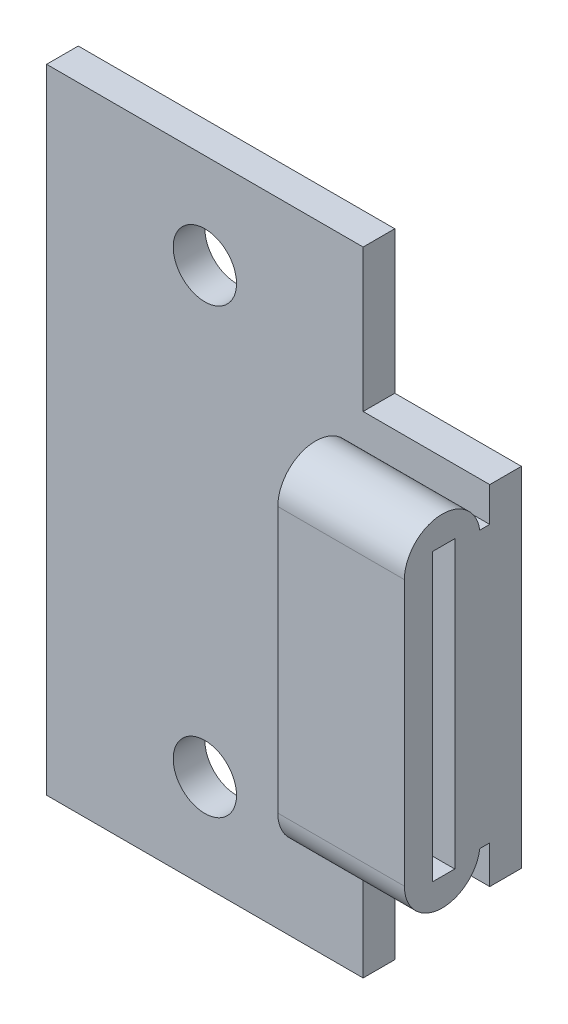
SolidWorks part; units mm, degrees
ref_plane "Front Plane" through (0, 0, 0) normal (0, 0, 1) x (1, 0, 0)
ref_plane "Top Plane" through (0, 0, 0) normal (0, 1, 0) x (1, 0, 0)
ref_plane "Right Plane" through (0, 0, 0) normal (1, 0, 0) x (0, 0, -1)
other "Configuration Table"
sketch "Sketch1" plane through (0, 0, 0) normal (0, 0, 1) x (1, 0, 0)
  line L0 (0, 7) -> (0, -7) construction
  line L1 (-5, 10) -> (5, 10)
  line L2 (-5, 10) -> (-5, -10)
  line L3 (-5, -10) -> (5, -10)
  line L4 (5, 10) -> (5, 5.5)
  line L5 (-5, 10) -> (5, -10) construction
  line L6 (-5, -10) -> (5, 10) construction
  line L11 (9, 5.5) -> (9, -5.5)
  line L12 (1, 5.5) -> (9, -5.5) construction
  line L13 (1, -5.5) -> (9, 5.5) construction
  line L14 (5, 5.5) -> (9, 5.5)
  line L15 (5, -5.5) -> (5, -10)
  line L16 (5, -5.5) -> (9, -5.5)
  circle A4 centre (0, 7) radius 1
  circle A5 centre (0, -7) radius 1
  point P0 (0, 0)
  point P6 (0, 0)
  point P11 (5, 0)
  dimension "D5" = 7
  dimension "D6" = 2
  dimension "D7" = 2
  dimension "D1" = 10
  dimension "D2" = 20
  dimension "D3" = 14
  dimension "D4" = 5
  dimension "D8" = 11
  dimension "D9" = 4
extrude "Boss-Extrude1" add sketch "Sketch1" along normal blind 1
sketch "Sketch2" plane through (0, 0, 1) normal (0, 0, 1) x (1, 0, 0)
  line L0 (5, 5.5) -> (5, 10) construction
  line L1 (9, 5.5) -> (5, 5.5)
  line L2 (9, 5.5) -> (9, -5.5)
  line L3 (9, -5.5) -> (5, -5.5)
  line L4 (5, 5.5) -> (5, -5.5)
  line L5 (9, 5.5) -> (5, -5.5) construction
  line L6 (9, -5.5) -> (5, 5.5) construction
  line L7 (9, -5.5) -> (9, 5.5) construction
  line L8 (9, 5.5) -> (5, 5.5) construction
  point P0 (7, 0)
extrude "Boss-Extrude2" add sketch "Sketch2" along normal blind 3
sketch "Sketch3" plane through (9, 0, 0) normal (1, 0, 0) x (0, 0, -1)
  line L0 (-2.5, 5.5) -> (-2.5, -5.5) construction
  line L1 (-4, 5.5) -> (0, 5.5) construction
  line L2 (-4, -5.5) -> (0, -5.5) construction
  line L3 (-4, -5.5) -> (-4, 5.5) construction
  line L4 (-2.5, 4.2479) -> (-2.5, -4.1397) construction
  line L5 (-1.3037, 4.2479) -> (-1.3037, -4.1397)
  line L6 (-3.6963, 4.2479) -> (-3.6963, -4.1397)
  line L8 (-1, -5.5) -> (-4, -5.5)
  line L9 (-1, -5.5) -> (-1, 5.5)
  line L10 (-1, 5.5) -> (-4, 5.5)
  line L11 (-4, -5.5) -> (-4, 5.5)
  line L12 (-1, -5.5) -> (-4, 5.5) construction
  line L13 (-1, 5.5) -> (-4, -5.5) construction
  arc A0 (-1.3037, 4.2479) -> (-3.6963, 4.2479) centre (-2.5, 4.2479) ccw
  arc A1 (-3.6963, -4.1397) -> (-1.3037, -4.1397) centre (-2.5, -4.1397) ccw
  point P10 (-2.5, 0.0541)
  point P15 (-2.5, 0)
  dimension "D1" = 1.5
extrude "Cut-Extrude1" cut sketch "Sketch3" against normal blind 10
sketch "Sketch4" plane through (9, 0, 0) normal (1, 0, 0) x (0, 0, -1)
  line L1 (-2.8087, 4.5726) -> (-2.1052, 4.5726)
  line L2 (-2.8087, 4.5726) -> (-2.8087, -4.4644)
  line L3 (-2.8087, -4.4644) -> (-2.1052, -4.4644)
  line L4 (-2.1052, 4.5726) -> (-2.1052, -4.4644)
  line L5 (-2.8087, 4.5726) -> (-2.1052, -4.4644) construction
  line L6 (-2.8087, -4.4644) -> (-2.1052, 4.5726) construction
  point P0 (-2.4569, 0.0541)
extrude "Cut-Extrude2" cut sketch "Sketch4" against normal blind 3
sketch "Sketch5" plane through (9, 0, 0) normal (1, 0, 0) x (0, 0, -1)
  line L0 (-1.3037, -4.1397) -> (-1.3037, 4.2479) construction
  line L1 (-1.6073, -4.302) -> (-1, -4.302)
  line L2 (-1.6073, -4.302) -> (-1.6073, 4.4103)
  line L3 (-1.6073, 4.4103) -> (-1, 4.4103)
  line L4 (-1, -4.302) -> (-1, 4.4103)
  line L5 (-1.6073, -4.302) -> (-1, 4.4103) construction
  line L6 (-1.6073, 4.4103) -> (-1, -4.302) construction
  line L7 (-1, -5.5) -> (-1, 5.5) construction
  point P0 (-1.3037, 0.0541)
extrude "Boss-Extrude3" add sketch "Sketch5" against normal blind 4
